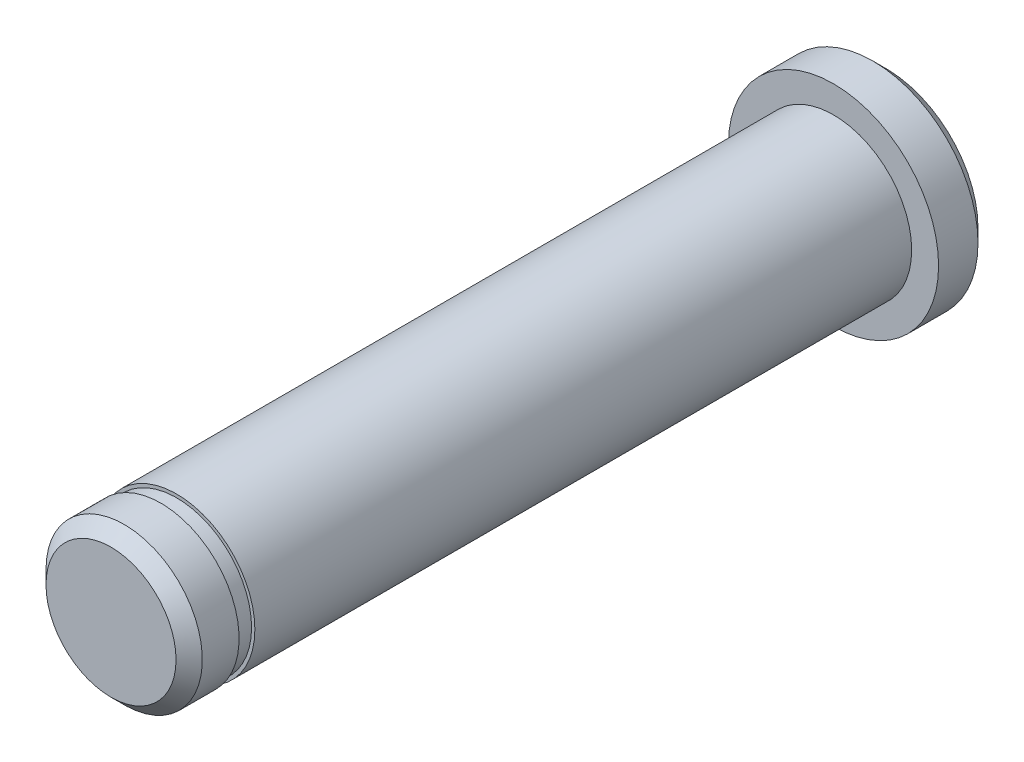
from build123d import *

# Parameters (mm, degrees)
SKETCH1_R           = 4
BOSS_EXTRUDE1_DEPTH = 2
SKETCH3_R           = 2.975
BOSS_EXTRUDE2_DEPTH = 25
SKETCH4_R           = 2.85
BOSS_EXTRUDE3_DEPTH = 0.6
SKETCH5_R           = 2.975
BOSS_EXTRUDE4_DEPTH = 1.9
CHAMFER1_SIZE       = 0.5


with BuildPart() as part:
    # Sketch1 → Boss-Extrude1 (new body)
    with BuildSketch(Plane.XY):
        Circle(SKETCH1_R)
    extrude(amount=BOSS_EXTRUDE1_DEPTH)

    # Sketch3 → Boss-Extrude2 (add)
    with BuildSketch(Plane.XY.offset(2)):
        Circle(SKETCH3_R)
    extrude(amount=BOSS_EXTRUDE2_DEPTH)

    # Sketch4 → Boss-Extrude3 (add)
    with BuildSketch(Plane.XY.offset(27)):
        Circle(SKETCH4_R)
    extrude(amount=BOSS_EXTRUDE3_DEPTH)

    # Sketch5 → Boss-Extrude4 (add)
    with BuildSketch(Plane.XY.offset(27.6)):
        Circle(SKETCH5_R)
    extrude(amount=BOSS_EXTRUDE4_DEPTH)

    # Chamfer1
    chamfer1_edges = [part.edges().sort_by_distance(p)[0] for p in [
        (-2.975, 0, 29.5),
        (-4, 0, 0),
    ]]
    chamfer(chamfer1_edges, length=CHAMFER1_SIZE)


solid = part.part
